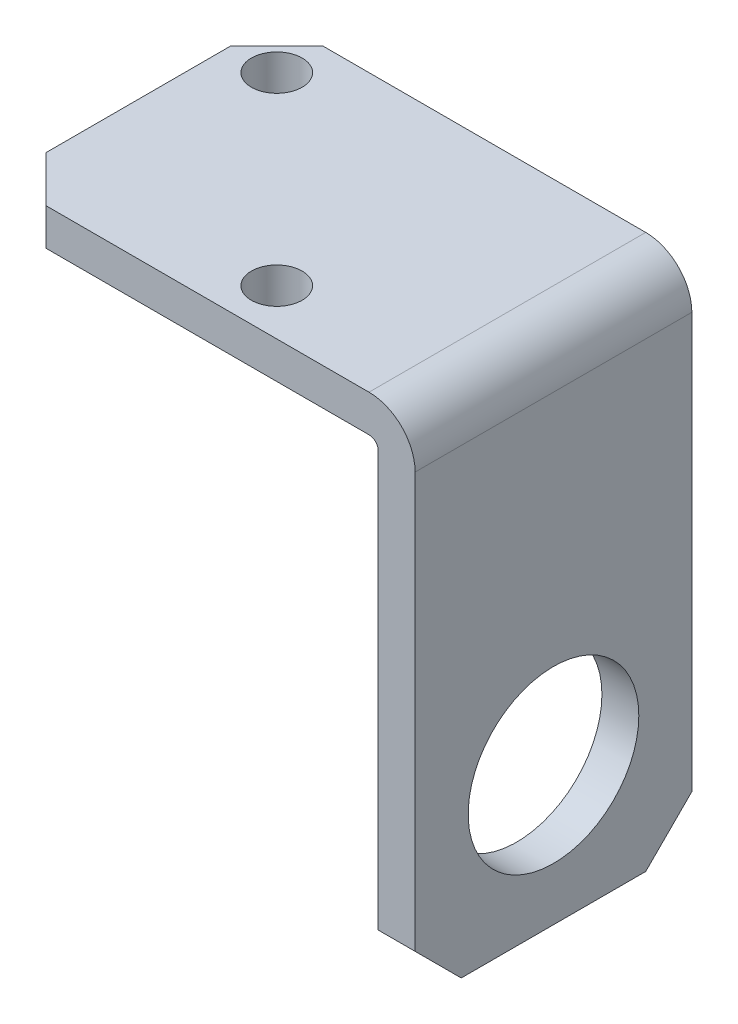
from build123d import *

# Parameters (mm, degrees)
EXTRUDE_1_DEPTH     = 30
SKETCH_3_R          = 9.25
CUT_EXTRUDE_1_DEPTH = 30
SKETCH_4_R          = 2.75
CUT_EXTRUDE_2_DEPTH = 30
CHAMFER_1_SIZE      = 5


with BuildPart() as part:
    # 草图1 → 凸台-拉伸1 (new body)
    with BuildSketch(Plane.XY):
        with BuildLine():
            Line((0, 0), (40, 0))
            ThreePointArc((40, 0), (43.535533906, -1.464466094), (45, -5))
            Line((45, -5), (45, -55))
            Line((45, -55), (41, -55))
            Line((41, -55), (41, -5))
            ThreePointArc((41, -5), (40.707106781, -4.292893219), (40, -4))
            Line((40, -4), (0, -4))
            Line((0, -4), (0, 0))
        make_face()
    extrude(amount=EXTRUDE_1_DEPTH)

    # 草图3 → 切除-拉伸1 (cut)
    with BuildSketch(Plane(origin=(45, 0, 0), x_dir=(0, 0, -1), z_dir=(1, 0, 0))):
        with Locations((-15, -40)):
            Circle(SKETCH_3_R)
    extrude(amount=-CUT_EXTRUDE_1_DEPTH, mode=Mode.SUBTRACT)

    # 草图4 → 切除-拉伸2 (cut)
    with BuildSketch(Plane(origin=(0, 0, 0), x_dir=(1, 0, 0), z_dir=(0, 1, 0))):
        with Locations(Location((5, -5, 0), (0, 0, 180))):
            Circle(SKETCH_4_R)
        with Locations(Location((25, -25, 0), (0, 0, 180))):
            Circle(SKETCH_4_R)
    extrude(amount=-CUT_EXTRUDE_2_DEPTH, mode=Mode.SUBTRACT)

    # 倒角1
    chamfer_1_edges = [part.edges().sort_by_distance(p)[0] for p in [
        (43, -55, 0),
        (0, -2, 30),
        (43, -55, 30),
        (0, -2, 0),
    ]]
    chamfer(chamfer_1_edges, length=CHAMFER_1_SIZE)


solid = part.part
